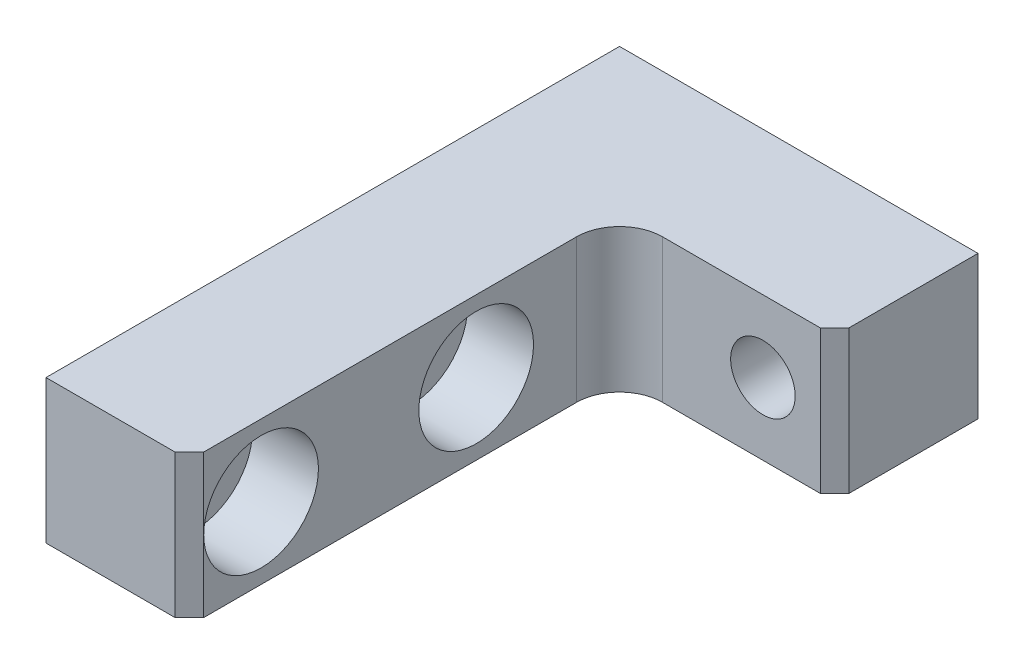
SolidWorks part; units mm, degrees
material "A6061"
ref_plane "前基準面" through (0, 0, 0) normal (0, 0, 1) x (1, 0, 0)
ref_plane "上基準面" through (0, 0, 0) normal (0, 1, 0) x (1, 0, 0)
ref_plane "右基準面" through (0, 0, 0) normal (1, 0, 0) x (0, 0, -1)
sketch "草图1" plane through (0, 0, 0) normal (0, 1, 0) x (1, 0, 0)
  line L1 (-12.5, -20) -> (12.5, -20)
  line L2 (-12.5, -20) -> (-12.5, 20)
  line L3 (-12.5, 20) -> (12.5, 20)
  line L4 (12.5, -20) -> (12.5, 20)
  line L5 (-12.5, -20) -> (12.5, 20) construction
  line L6 (-12.5, 20) -> (12.5, -20) construction
  point P0 (0, 0)
  dimension "D1" = 25
  dimension "D2" = 40
extrude "凸台-拉伸1" add sketch "草图1" along normal mid plane 10
sketch "草图2" plane through (0, 5, 0) normal (0, 1, 0) x (1, 0, 0)
  line L0 (12.5, 20) -> (-12.5, 20) construction
  line L1 (12.5, -20) -> (-2.5, -20)
  line L2 (12.5, -20) -> (12.5, 10)
  line L3 (12.5, 10) -> (0.5, 10)
  line L4 (-2.5, -20) -> (-2.5, 7)
  line L5 (-12.5, 20) -> (-12.5, -20) construction
  arc A0 (0.5, 10) -> (-2.5, 7) centre (0.5, 7) ccw
  dimension "D3" = 3
  dimension "D1" = 10
  dimension "D2" = 10
extrude "切除-拉伸1" cut sketch "草图2" against normal up to surface (10 mm away) up to face at (0, -5, 0)
chamfer "倒角1" distance 1 angle 45 2 edges at (-2.5, 0, 20) (12.5, 0, -10)
hole_wizard "打孔尺寸(%根据)内六角圆柱头螺钉的类型1" positions "草图3" profile "草图4" counterbore size "M4" standard "GB" end condition through all
sketch "草图3" plane through (-2.5, 0, 0) normal (1, 0, 0) x (0, 0, -1)
  line L0 (-20, -5) -> (-20, 5) construction
  point P0 (-15, 0)
  point P2 (0, 0)
  dimension "D1" = 5
  dimension "D2" = 15
sketch "草图4" plane through (-2.5, 0, 15) normal (0, 1, 0) x (0, 0, -1)
  line L0 (0, 0) -> (0, 10)
  line L1 (0, 10) -> (2.25, 10)
  line L3 (2.25, 10) -> (2.25, 4.6)
  line L4 (2.25, 4.6) -> (4, 4.6)
  line L5 (4, 4.6) -> (4, 0)
  line L7 (4, 0) -> (0, 0)
  line L11 (0, -6.35) -> (0, 107.95) construction
  dimension "通孔孔直径" = 4.5
  dimension "通孔孔深度" = 10
  dimension "柱形沉头孔直径" = 8
  dimension "柱形沉头孔深度" = 4.6
hole_wizard "M4 间隙孔1" positions "草图5" profile "草图6" hole size "M4" standard "GB" end condition through all
sketch "草图5" plane through (0, 0, -10) normal (0, 0, 1) x (1, 0, 0)
  line L0 (12.5, 5) -> (12.5, -5) construction
  point P0 (7.5, 0)
  dimension "D1" = 5
sketch "草图6" plane through (7.5, 0, -10) normal (1, 0, 0) x (0, -1, 0)
  line L0 (0, 0) -> (0, 10)
  line L1 (0, 10) -> (2.25, 10)
  line L2 (2.25, 10) -> (2.25, 0)
  line L5 (2.25, 0) -> (0, 0)
  line L11 (0, -6.35) -> (0, 107.95) construction
  dimension "通孔孔直径" = 4.5
  dimension "通孔孔深度" = 10
